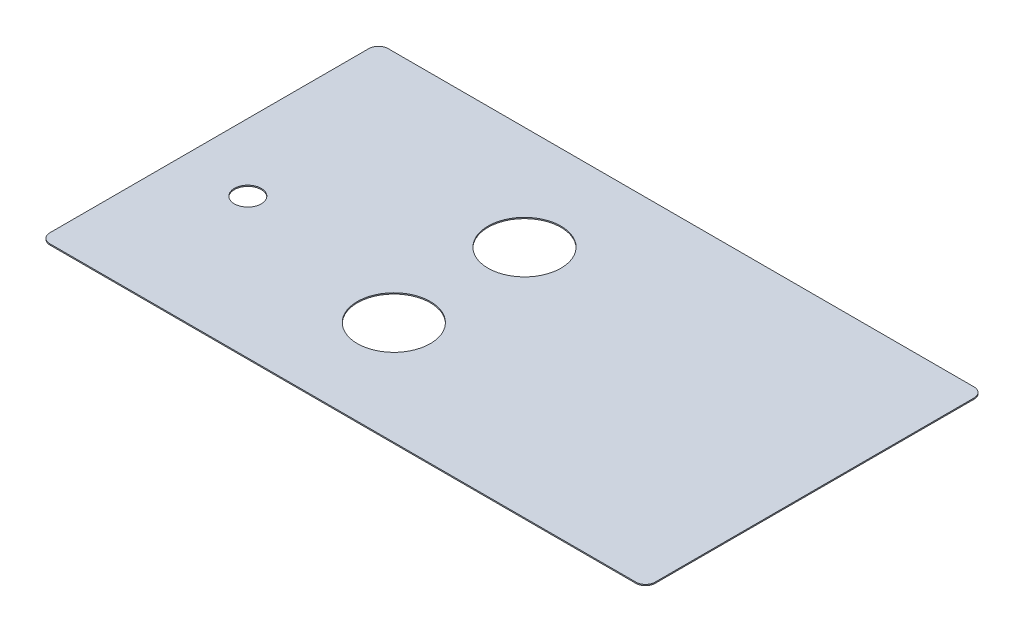
from build123d import *

# Parameters (mm, degrees)
SKETCH1_R           = 19
SKETCH1_R_2         = 7
BOSS_EXTRUDE1_DEPTH = 0.3


with BuildPart() as part:
    # Sketch1 → Boss-Extrude1 (new, symmetric)
    with BuildSketch(Plane(origin=(0, 0, 0), x_dir=(1, 0, 0), z_dir=(0, 1, 0))):
        with BuildLine():
            Line((-130, 83), (-130, -83))
            ThreePointArc((-130, -83), (-128.535533906, -86.535533906), (-125, -88))
            Line((-125, -88), (180, -88))
            ThreePointArc((180, -88), (183.535533906, -86.535533906), (185, -83))
            Line((185, -83), (185, 83))
            ThreePointArc((185, 83), (183.535533906, 86.535533906), (180, 88))
            Line((180, 88), (-125, 88))
            ThreePointArc((-125, 88), (-128.535533906, 86.535533906), (-130, 83))
        make_face()
        with Locations(Location((0, 34, 0), (0, 0, 270))):
            Circle(SKETCH1_R, mode=Mode.SUBTRACT)
        with Locations(Location((0, -34, 0), (0, 0, 270))):
            Circle(SKETCH1_R, mode=Mode.SUBTRACT)
        with Locations(Location((-95, -15, 0), (0, 0, 270))):
            Circle(SKETCH1_R_2, mode=Mode.SUBTRACT)
    extrude(amount=BOSS_EXTRUDE1_DEPTH, both=True)


solid = part.part
